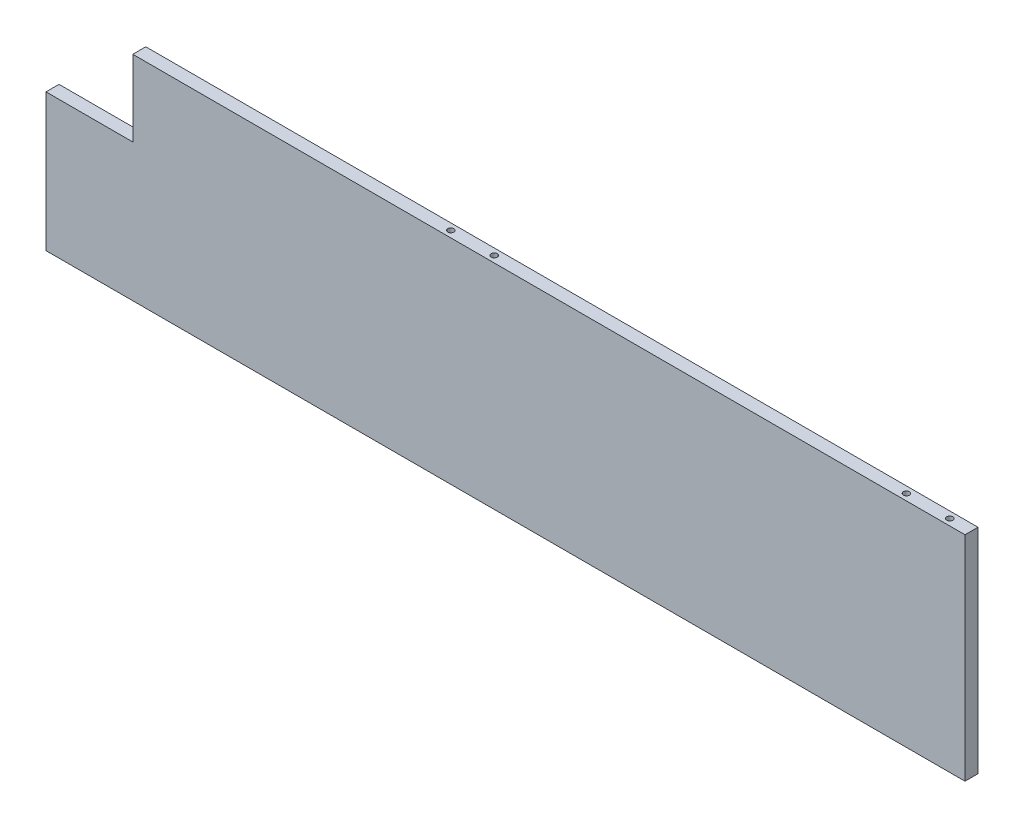
from build123d import *

# Parameters (mm, degrees)
BOSS_EXTRUDE1_DEPTH    = 30
M16_TAPPED_HOLE1_D     = 14
M16_TAPPED_HOLE1_DEPTH = 45
M16_TAPPED_HOLE1_TIP   = 4.206024333


with BuildPart() as part:
    # Sketch1 → Boss-Extrude1 (new body)
    with BuildSketch(Plane.XY):
        Polygon((0, 317), (200, 317), (200, 492), (2118, 492), (2118, 0), (0, 0), align=None)
    extrude(amount=BOSS_EXTRUDE1_DEPTH)

    # M16 Tapped Hole1
    with Locations(Plane(origin=(918, 492, 15), x_dir=(0, 0, 1), z_dir=(0, 1, 0))):
        with Locations((0, 0), (0, 100), (0, 1150), (0, 1050)):
            Hole(M16_TAPPED_HOLE1_D / 2, depth=M16_TAPPED_HOLE1_DEPTH)
            with Locations((0, 0, -(M16_TAPPED_HOLE1_DEPTH + M16_TAPPED_HOLE1_TIP / 2))):  # 118° drill point
                Cone(0, M16_TAPPED_HOLE1_D / 2, M16_TAPPED_HOLE1_TIP, mode=Mode.SUBTRACT)


solid = part.part
